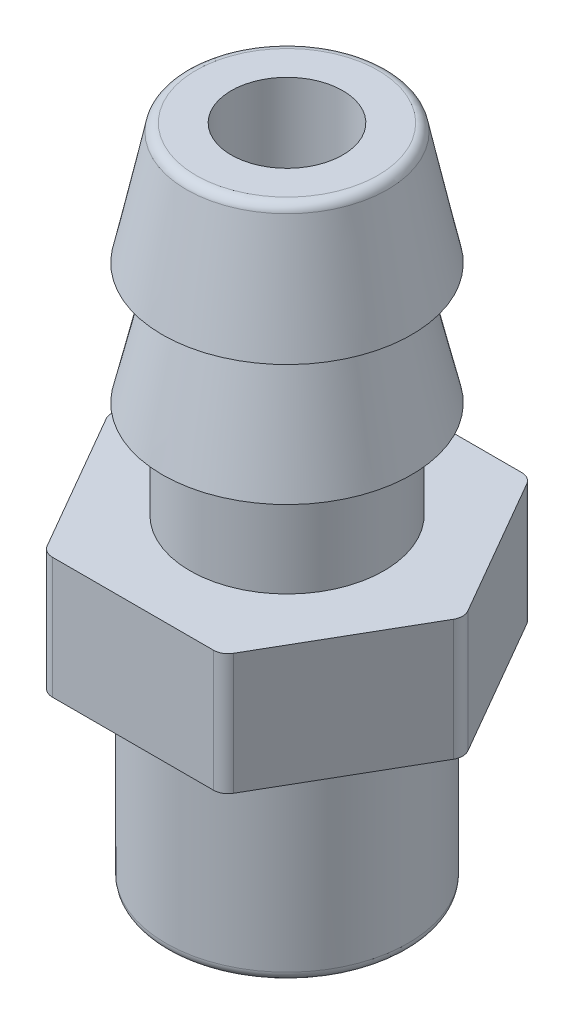
SolidWorks part; units mm, degrees
material "OTHER"
ref_plane "Front Plane" through (0, 0, 0) normal (0, 0, 1) x (1, 0, 0)
ref_plane "Top Plane" through (0, 0, 0) normal (0, 1, 0) x (1, 0, 0)
ref_plane "Right Plane" through (0, 0, 0) normal (1, 0, 0) x (0, 0, -1)
sketch "Sketch1" plane through (0, 0, 0) normal (0, 1, 0) x (1, 0, 0)
  line L1 (3.6662, 0) -> (1.8331, 3.175)
  line L2 (1.8331, 3.175) -> (-1.8331, 3.175)
  line L3 (-1.8331, 3.175) -> (-3.6662, 0)
  line L4 (-3.6662, 0) -> (-1.8331, -3.175)
  line L5 (-1.8331, -3.175) -> (1.8331, -3.175)
  line L6 (1.8331, -3.175) -> (3.6662, 0)
  circle A0 centre (0, 0) radius 3.175 construction
  dimension "D1" = 6.35
extrude "Boss-Extrude1" add sketch "Sketch1" along normal blind 2.5
sketch "Sketch2" plane through (0, 2.5, 0) normal (0, 1, 0) x (1, 0, 0)
  circle A0 centre (0, 0) radius 2
  dimension "D1" = 4
extrude "Boss-Extrude2" add sketch "Sketch2" along normal blind 2
sketch "Sketch3" plane through (0, 4.5, 0) normal (0, 1, 0) x (1, 0, 0)
  circle A0 centre (0, 0) radius 2.57
  dimension "D1" = 5.14
extrude "Boss-Extrude3" add sketch "Sketch3" along normal blind 2.5 draft 13
sketch "Sketch4" plane through (0, 7, 0) normal (0, 1, 0) x (1, 0, 0)
  circle A1 centre (0, 0) radius 2.57
  circle A2 centre (0, 0) radius 2.57
  dimension "D1" = 0
extrude "Boss-Extrude4" add sketch "Sketch4" along normal blind 2.5 draft 12
sketch "Sketch5" plane through (0, 0, 0) normal (0, -1, 0) x (1, 0, 0)
  circle A0 centre (0, 0) radius 2.5
  circle A1 centre (0, 0) radius 1.15
  dimension "D1" = 5
  dimension "D2" = 1.35
extrude "Boss-Extrude5" add sketch "Sketch5" along normal blind 4.1
sketch "Sketch6" plane through (0, 0, 0) normal (0, -1, 0) x (1, 0, 0)
  circle A2 centre (0, 0) radius 1.15
  dimension "D1" = 2.3
extrude "Cut-Extrude1" cut sketch "Sketch6" against normal through all
fillet "Fillet1" radius 0.3 6 edges at (-1.8331, 1.25, 3.175) (-3.6662, 1.25, 0) (-1.8331, 1.25, -3.175) (1.8331, 1.25, 3.175) (3.6662, 1.25, 0) (1.8331, 1.25, -3.175)
fillet "Fillet2" radius 0.2 2 edges at (0, -4.1, -2.5) (0, 9.5, 2.0386)
